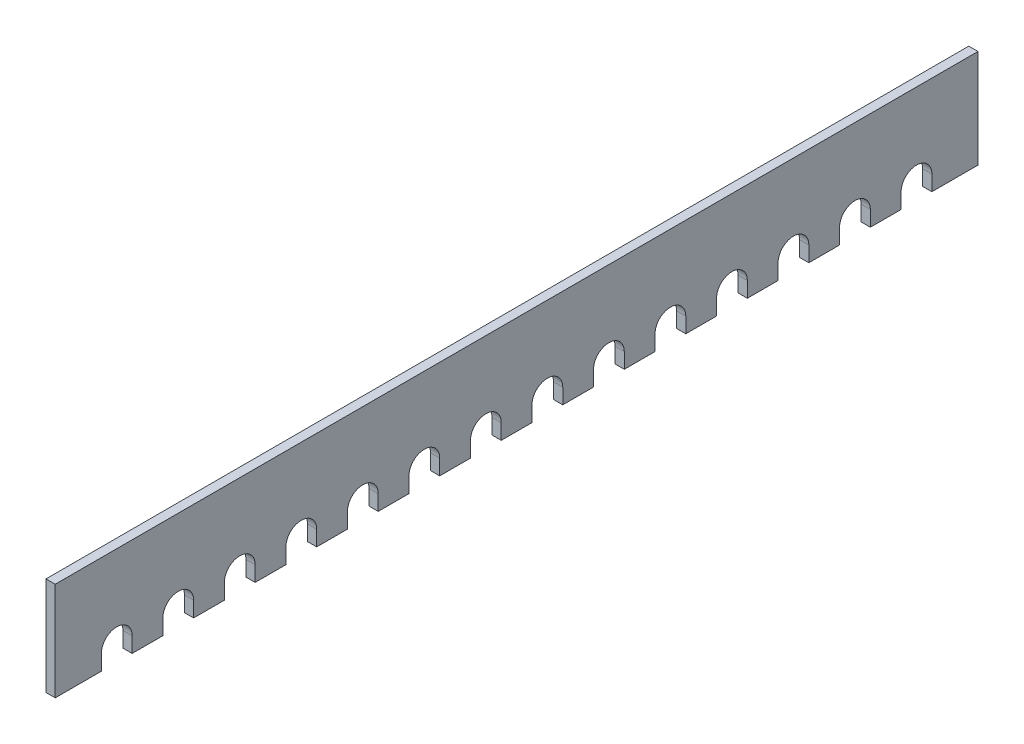
from build123d import *

# Parameters (mm, degrees)
SKETCH1_W           = 3
SKETCH1_H           = 32
EXTRUDE_THIN1_DEPTH = 300
CUT_EXTRUDE1_DEPTH  = 302.716754589
LPATTERN1_COUNT     = 14
LPATTERN1_PITCH     = 20


with BuildPart() as part:
    # Sketch1 → Extrude-Thin1 (new body)
    with BuildSketch(Plane.XY):
        with Locations((-1.5, -16)):
            Rectangle(SKETCH1_W, SKETCH1_H)
    extrude(amount=EXTRUDE_THIN1_DEPTH)

    # Sketch2 → Cut-Extrude1 (cut, through all)
    with BuildSketch(Plane(origin=(0, 0, 0), x_dir=(0, 0, -1), z_dir=(1, 0, 0))):
        with BuildLine():
            Line((-275, -27), (-275, -32))
            Line((-275, -32), (-285, -32))
            Line((-285, -32), (-285, -27))
            ThreePointArc((-285, -27), (-280, -22), (-275, -27))
        make_face()
    cut_extrude1 = extrude(amount=-CUT_EXTRUDE1_DEPTH, mode=Mode.SUBTRACT)

    # LPattern1: Cut-Extrude1 ×14
    with Locations(*[(0, 0, -i * LPATTERN1_PITCH) for i in range(1, LPATTERN1_COUNT)]):
        add(cut_extrude1, mode=Mode.SUBTRACT)


solid = part.part
